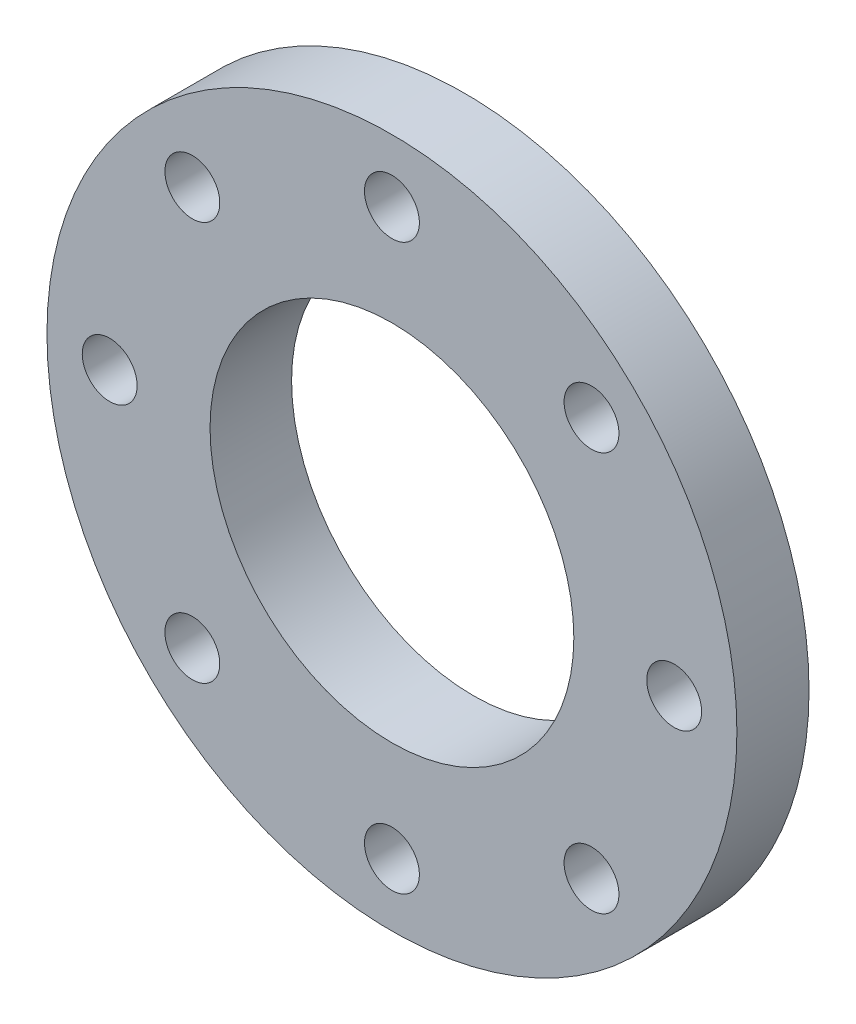
from build123d import *

# Parameters (mm, degrees)
SKETCH1_R               = 110
SKETCH1_R_2             = 8.75
BOSS_EXTRUDE1_DEPTH     = 26
CUT_EXTRUDE1_DEPTH      = 158.721273137
CUT_EXTRUDE1_DEPTH_BACK = 158.721273137
SKETCH4_R               = 58


with BuildPart() as part:
    # Sketch1 → Boss-Extrude1 (new body)
    with BuildSketch(Plane.XY):
        with Locations(Location((0, 0, 0), (0, 0, 180))):
            Circle(SKETCH1_R)
        with Locations(Location((0, 90, 0), (0, 0, 180))):
            Circle(SKETCH1_R_2, mode=Mode.SUBTRACT)
        with Locations(Location((63.639610307, 63.639610307, 0), (0, 0, 180))):
            Circle(SKETCH1_R_2, mode=Mode.SUBTRACT)
        with Locations(Location((90, 0, 0), (0, 0, 180))):
            Circle(SKETCH1_R_2, mode=Mode.SUBTRACT)
        with Locations(Location((63.639610307, -63.639610307, 0), (0, 0, 180))):
            Circle(SKETCH1_R_2, mode=Mode.SUBTRACT)
        with Locations(Location((0, -90, 0), (0, 0, 180))):
            Circle(SKETCH1_R_2, mode=Mode.SUBTRACT)
        with Locations(Location((-63.639610307, -63.639610307, 0), (0, 0, 180))):
            Circle(SKETCH1_R_2, mode=Mode.SUBTRACT)
        with Locations(Location((-90, 0, 0), (0, 0, 180))):
            Circle(SKETCH1_R_2, mode=Mode.SUBTRACT)
        with Locations(Location((-63.639610307, 63.639610307, 0), (0, 0, 180))):
            Circle(SKETCH1_R_2, mode=Mode.SUBTRACT)
    extrude(amount=BOSS_EXTRUDE1_DEPTH)

    # Sketch3 → Cut-Revolve1 (revolve, cut)
    with BuildSketch(Plane(origin=(0, 0, 0), x_dir=(1, 0, 0), z_dir=(0, 1, 0)), mode=Mode.PRIVATE) as cut_revolve1_sk:
        Polygon((81, 0), (79, 0), (81, -3), (110, -3), (110, 0), align=None)
    revolve(cut_revolve1_sk.sketch.rotate(Axis((0, 0, 0), (0, 0, 1)), 180), axis=Axis((0, 0, 0), (0, 0, 1)), mode=Mode.SUBTRACT)

    # Sketch4 → Cut-Extrude1 (cut, two sides: drawn at the far end of the back side and taken through both)
    with BuildSketch(Plane(origin=(0, 0, 0), x_dir=(-1, 0, 0), z_dir=(0, 0, -1)).offset(-CUT_EXTRUDE1_DEPTH_BACK)):
        Circle(SKETCH4_R)
    extrude(amount=CUT_EXTRUDE1_DEPTH + CUT_EXTRUDE1_DEPTH_BACK, mode=Mode.SUBTRACT)


solid = part.part
